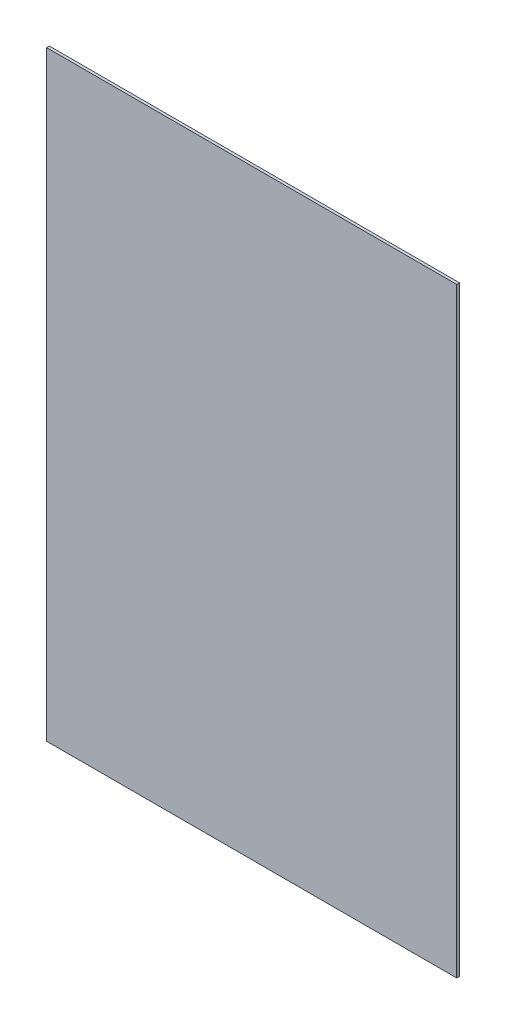
from build123d import *

# Parameters (mm, degrees)
SKETCH_1_W      = 745
SKETCH_1_H      = 1091
EXTRUDE_1_DEPTH = 5


with BuildPart() as part:
    # 草图1 → 凸台-拉伸1 (new body)
    with BuildSketch(Plane.XY):
        Rectangle(SKETCH_1_W, SKETCH_1_H)
    extrude(amount=EXTRUDE_1_DEPTH)


solid = part.part
